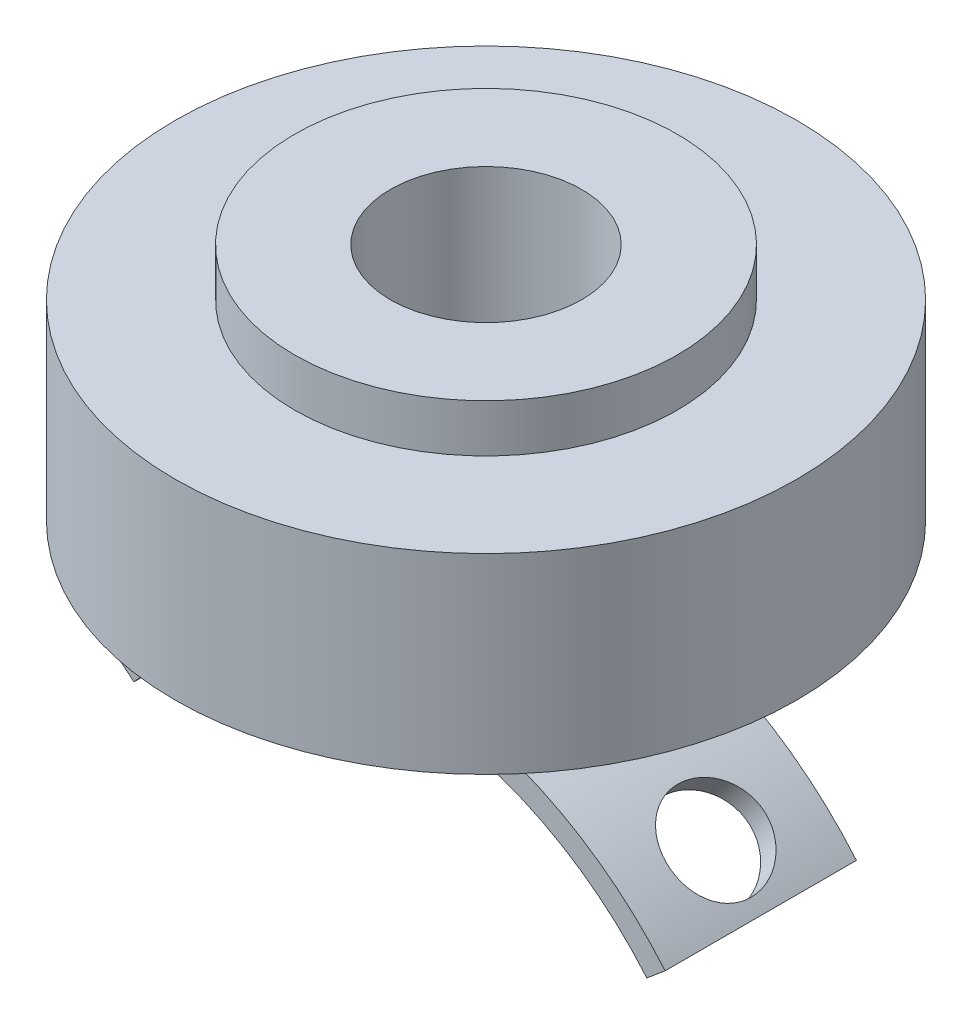
SolidWorks part; units mm, degrees
ref_plane "Front Plane" through (0, 0, 0) normal (0, 0, 1) x (1, 0, 0)
ref_plane "Top Plane" through (0, 0, 0) normal (0, 1, 0) x (1, 0, 0)
ref_plane "Right Plane" through (0, 0, 0) normal (1, 0, 0) x (0, 0, -1)
other "Configuration Table"
sketch "Sketch4" plane through (0, 0, 0) normal (0, 0, 1) x (1, 0, 0)
  line L0 (-26.8116, 22.4976) -> (-28.7267, 24.1045)
  line L1 (26.8116, 22.4976) -> (28.7267, 24.1045)
  line L2 (0, 75.012) -> (0, 35) construction
  arc A0 (26.8116, 22.4976) -> (-26.8116, 22.4976) centre (0, 0) ccw
  arc A1 (28.7267, 24.1045) -> (-28.7267, 24.1045) centre (0, 0) ccw
  dimension "D1" = 70
  dimension "D2" = 75
  dimension "D3" = 50
  dimension "D4" = 50
extrude "Boss-Extrude4" add sketch "Sketch4" along normal blind 20
ref_plane "Plane2" through (0, 0, 10) normal (0, 0, 1) x (1, 0, 0)
ref_plane "Plane4" through (0, 40.5, 0) normal (0, 1, 0) x (1, 0, 0)
sketch "Sketch8" plane through (0, 40.5, 0) normal (0, 1, 0) x (1, 0, 0)
  line L0 (28.7267, 0) -> (-28.7267, 0) construction
  circle A0 centre (0, -10) radius 10
  dimension "D2" = 20
  dimension "D1" = 10
extrude "Boss-Extrude5" add sketch "Sketch8" against normal up to body
sketch "Sketch9" plane through (0, 40.5, 0) normal (0, 1, 0) x (1, 0, 0)
  circle A0 centre (0, -10) radius 20
  dimension "D1" = 40
extrude "Boss-Extrude6" add sketch "Sketch9" along normal blind 5 separate body
sketch "Sketch10" plane through (0, 45.5, 0) normal (0, 1, 0) x (1, 0, 0)
  circle A0 centre (0, -10) radius 32.5
  dimension "65" = 65
extrude "Boss-Extrude7" add sketch "Sketch10" along normal blind 20
sketch "Sketch11" plane through (0, 65.5, 0) normal (0, 1, 0) x (1, 0, 0)
  circle A0 centre (0, -10) radius 20
  dimension "D1" = 40
extrude "Boss-Extrude8" add sketch "Sketch11" along normal blind 5
sketch "Sketch12" plane through (0, 70.5, 0) normal (0, 1, 0) x (1, 0, 0)
  circle A0 centre (0, -10) radius 10
  dimension "D1" = 20
extrude "Cut-Extrude3" cut sketch "Sketch12" against normal blind 20 contours A0
cosmetic thread "Cosmetic Thread1" parameters "D2"=24
sketch "Sketch14" plane through (0, 0, 20) normal (0, 0, 1) x (1, 0, 0)
  line L0 (0, 0) -> (0, 37.5) construction
sketch "Sketch15" plane through (0, 0, 10) normal (0, 0, 1) x (1, 0, 0)
  line L0 (-17.6931, 21.0859) -> (-26.2782, 31.3171)
  line L1 (-26.2782, 31.3171) -> (-30.1084, 28.1031)
  line L2 (-30.1084, 28.1031) -> (-21.5234, 17.8719)
  line L3 (-21.5234, 17.8719) -> (-17.6931, 21.0859)
  line L4 (0, 0) -> (0, 37.5) construction
  dimension "D1" = 40
  dimension "D2" = 5
revolve "Cut-Revolve3" cut sketch "Sketch15" angle 360 about L0
cosmetic thread "Cosmetic Thread2" parameters "D2"=12
sketch "Sketch16" plane through (0, 0, 10) normal (0, 0, 1) x (1, 0, 0)
  line L0 (17.7926, 21.2044) -> (27.6372, 32.9367)
  line L1 (27.6372, 32.9367) -> (23.8069, 36.1506)
  line L2 (23.8069, 36.1506) -> (13.9624, 24.4184)
  line L3 (13.9624, 24.4184) -> (17.7926, 21.2044)
  line L4 (0, 0) -> (0, 37.5) construction
  dimension "D1" = 40
  dimension "D2" = 5
revolve "Cut-Revolve4" cut sketch "Sketch16" angle 360 about L0
